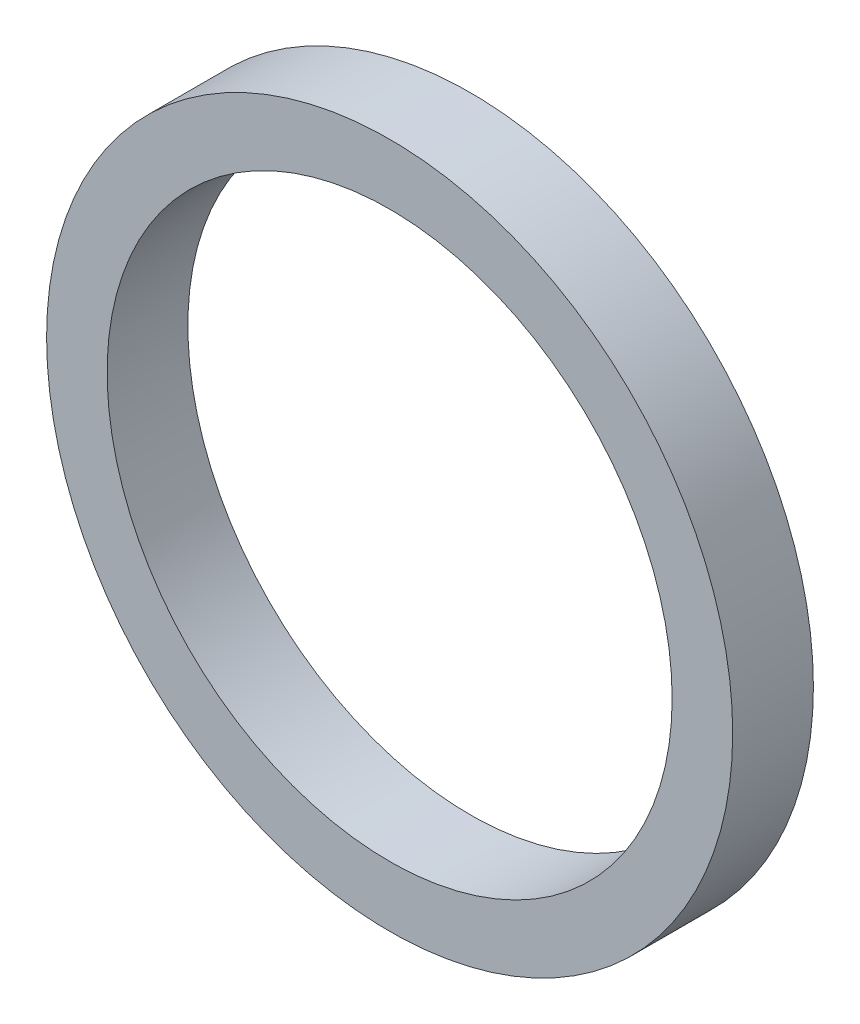
SolidWorks part; units mm, degrees
ref_plane "前视基准面" through (0, 0, 0) normal (0, 0, 1) x (1, 0, 0)
ref_plane "上视基准面" through (0, 0, 0) normal (0, 1, 0) x (1, 0, 0)
ref_plane "右视基准面" through (0, 0, 0) normal (1, 0, 0) x (0, 0, -1)
sketch "草图1" plane through (0, 0, 0) normal (0, 0, 1) x (1, 0, 0)
  circle A0 centre (0, 0) radius 17.5
  circle A1 centre (0, 0) radius 21.25
  dimension "D1" = 35
  dimension "D2" = 42.5
extrude "凸台-拉伸1" add sketch "草图1" along normal blind 5
